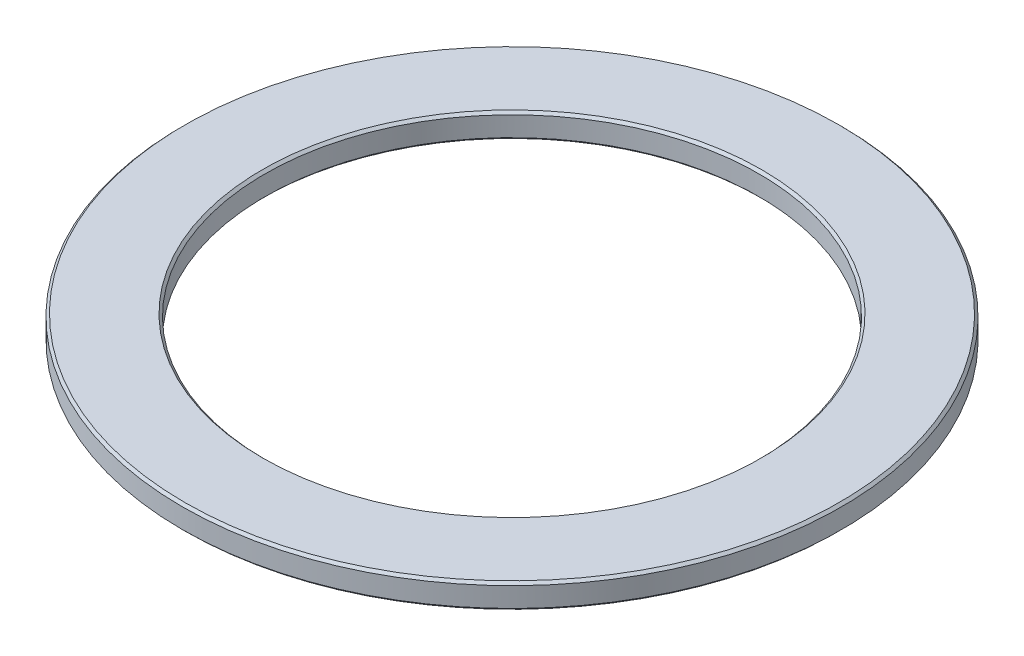
SolidWorks part; units mm, degrees
ref_plane "Front Plane" through (0, 0, 0) normal (0, 0, 1) x (1, 0, 0)
ref_plane "Top Plane" through (0, 0, 0) normal (0, 1, 0) x (1, 0, 0)
ref_plane "Right Plane" through (0, 0, 0) normal (1, 0, 0) x (0, 0, -1)
sketch "Sketch1" plane through (0, 0, 0) normal (0, 1, 0) x (1, 0, 0)
  circle A0 centre (0, 0) radius 40
  circle A1 centre (0, 0) radius 30
  dimension "D1" = 80
  dimension "D2" = 60
extrude "Boss-Extrude1" add sketch "Sketch1" along normal mid plane 3
chamfer "Chamfer1" distance 0.3 angle 45 4 edges at (0, -1.5, 40) (0, 1.5, 40) (0, -1.5, 30) (0, 1.5, 30)
